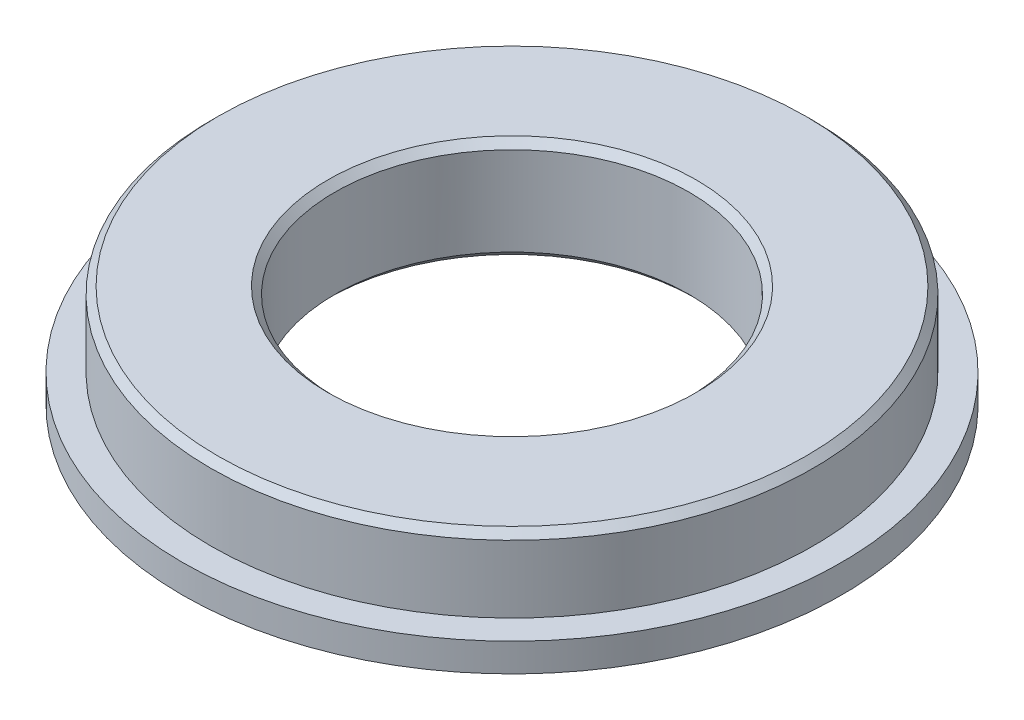
SolidWorks part; units mm, degrees
material "Q355"
ref_plane "Front Plane" through (0, 0, 0) normal (0, 0, 1) x (1, 0, 0)
ref_plane "Top Plane" through (0, 0, 0) normal (0, 1, 0) x (1, 0, 0)
ref_plane "Right Plane" through (0, 0, 0) normal (1, 0, 0) x (0, 0, -1)
sketch "Sketch1" plane through (0, 0, 0) normal (0, 0, 1) x (1, 0, 0)
  line L0 (0, 0) -> (0, 14.5) construction
  line L1 (25, 0) -> (46.5, 0)
  line L2 (46.5, 0) -> (46.5, 4)
  line L3 (46.5, 4) -> (42.5, 4)
  line L4 (42.5, 4) -> (42.5, 14.5)
  line L5 (42.5, 14.5) -> (25, 14.5)
  line L6 (25, 14.5) -> (25, 0)
  dimension "D1" = 4
  dimension "D2" = 14.5
  dimension "D3" = 93
  dimension "D4" = 85
  dimension "D5" = 50
revolve "Revolve1" add sketch "Sketch1" angle 360 about L0
hole_wizard "M4 Tapped Hole1" positions "Sketch2" profile "Sketch3" tap size "M4" standard "GB"
sketch "Sketch2" plane through (0, 0, 0) normal (0, -1, 0) x (-1, 0, 0)
  point P0 (0, -36.5)
  point P11 (-31.6099, -18.25)
  point P12 (-31.6099, 18.25)
  point P13 (0, 36.5)
  point P14 (31.6099, 18.25)
  point P15 (31.6099, -18.25)
  dimension "D1" = 36.5
  dimension "D2" = 6
sketch "Sketch3" plane through (0, 0, 36.5) normal (1, 0, 0) x (0, 0, -1)
  line L0 (0, 0) -> (0, 10.7914)
  line L1 (0, 10.7914) -> (1.65, 9.8)
  line L2 (1.65, 9.8) -> (1.65, 0)
  line L5 (1.65, 0) -> (0, 0)
  line L10 (0, 10.7914) -> (-1.65, 9.8) construction
  line L11 (0, -6.35) -> (0, 107.95) construction
  dimension "螺纹孔钻头直径" = 3.3
  dimension "螺纹孔钻头深度" = 9.8
  dimension "导头角度" = 118
cosmetic thread "Cosmetic thread 1" parameters "D1"=7.9, "D2"=4
cosmetic thread "Cosmetic thread 2" parameters "D1"=7.9, "D2"=4
cosmetic thread "Cosmetic thread 3" parameters "D1"=7.9, "D2"=4
cosmetic thread "Cosmetic thread 4" parameters "D1"=7.9, "D2"=4
cosmetic thread "Cosmetic thread 5" parameters "D1"=7.9, "D2"=4
cosmetic thread "Cosmetic thread 6" parameters "D1"=7.9, "D2"=4
chamfer "Chamfer1" distance 1 angle 45 3 edges at (0, 0, -25) (0, 14.5, -25) (0, 14.5, -42.5)
